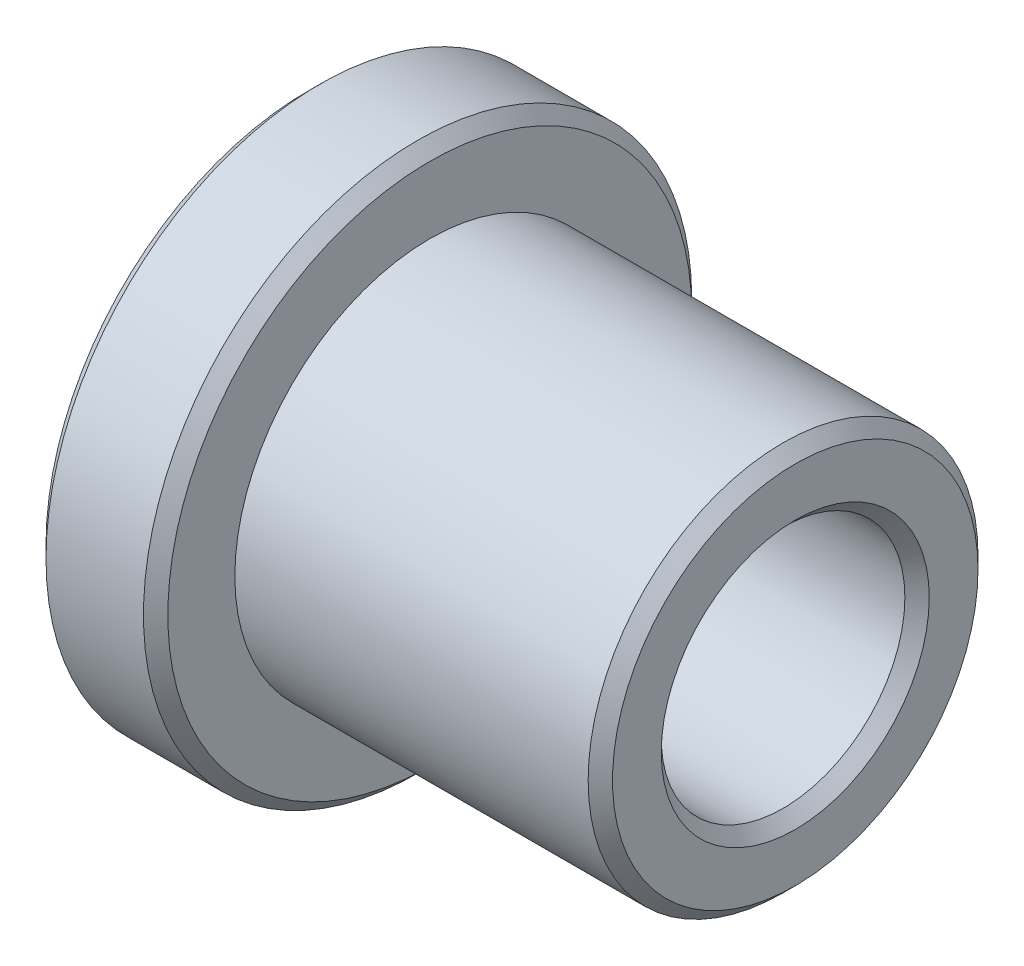
SolidWorks part; units mm, degrees
material "Q235A"
ref_plane "Front Plane" through (0, 0, 0) normal (0, 0, 1) x (1, 0, 0)
ref_plane "Top Plane" through (0, 0, 0) normal (0, 1, 0) x (1, 0, 0)
ref_plane "Right Plane" through (0, 0, 0) normal (1, 0, 0) x (0, 0, -1)
sketch "Sketch2" plane through (0, 0, 0) normal (0, 0, 1) x (1, 0, 0)
  line L0 (0, 0) -> (-49.6374, 0) construction
  line L1 (0, 10) -> (0, 16)
  line L2 (0, 16) -> (-30, 16)
  line L3 (-30, 16) -> (-30, 22.5)
  line L4 (-30, 22.5) -> (-40, 22.5)
  line L5 (-40, 22.5) -> (-40, 16)
  line L6 (-40, 16) -> (-45, 16)
  line L7 (-45, 16) -> (-45, 10)
  line L8 (-45, 10) -> (0, 10)
  dimension "D1" = 45
  dimension "D2" = 30
  dimension "D3" = 10
  dimension "D4" = 20
  dimension "D5" = 32
  dimension "D6" = 45
revolve "Revolve1" add sketch "Sketch2" angle 360 about L0
chamfer "Chamfer1" distance 1 angle 45 5 edges at (0, 0, -10) (0, 0, -16) (-30, 0, -22.5) (-40, 0, -22.5) (-45, 0, -10)
chamfer "Chamfer2" distance 3 angle 45 1 edges at (-45, 0, -16)
